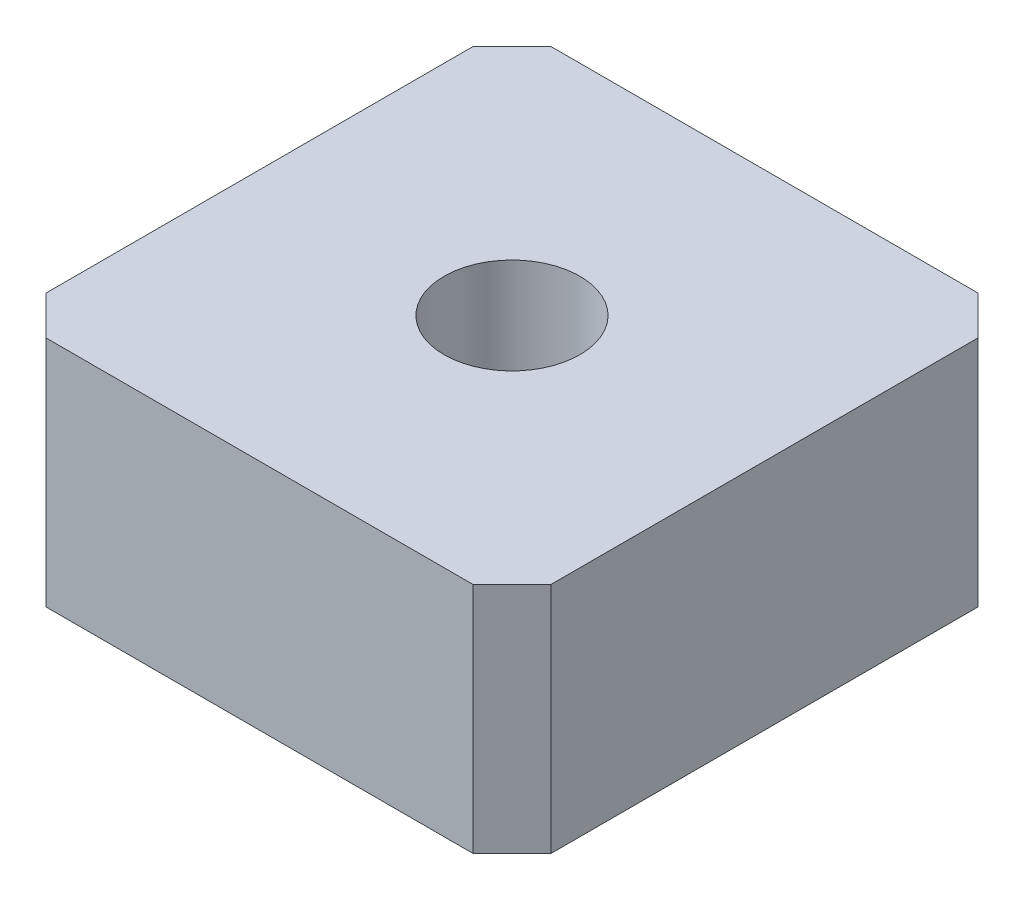
from build123d import *

# Parameters (mm, degrees)
SKETCH_1_W              = 13
SKETCH_1_H              = 13
EXTRUDE_1_DEPTH         = 6
HOLE_WIZARD_3_5_3_5_1_D = 3.5
CHAMFER_1_SIZE          = 1


with BuildPart() as part:
    # 草图1 → 凸台-拉伸1 (new body)
    with BuildSketch(Plane(origin=(0, 0, 0), x_dir=(1, 0, 0), z_dir=(0, 1, 0))):
        Rectangle(SKETCH_1_W, SKETCH_1_H)
    extrude(amount=EXTRUDE_1_DEPTH)

    # Ø3.5 (3.5) 直径孔1 (through all)
    with Locations(Plane(origin=(0, 6, 0), x_dir=(1, 0, 0), z_dir=(0, 1, 0))):
        with Locations((0, 0)):
            Hole(HOLE_WIZARD_3_5_3_5_1_D / 2)

    # 倒角1
    chamfer_1_edges = [part.edges().sort_by_distance(p)[0] for p in [
        (6.5, 3, 6.5),
        (-6.5, 3, 6.5),
        (-6.5, 3, -6.5),
        (6.5, 3, -6.5),
    ]]
    chamfer(chamfer_1_edges, length=CHAMFER_1_SIZE)


solid = part.part
